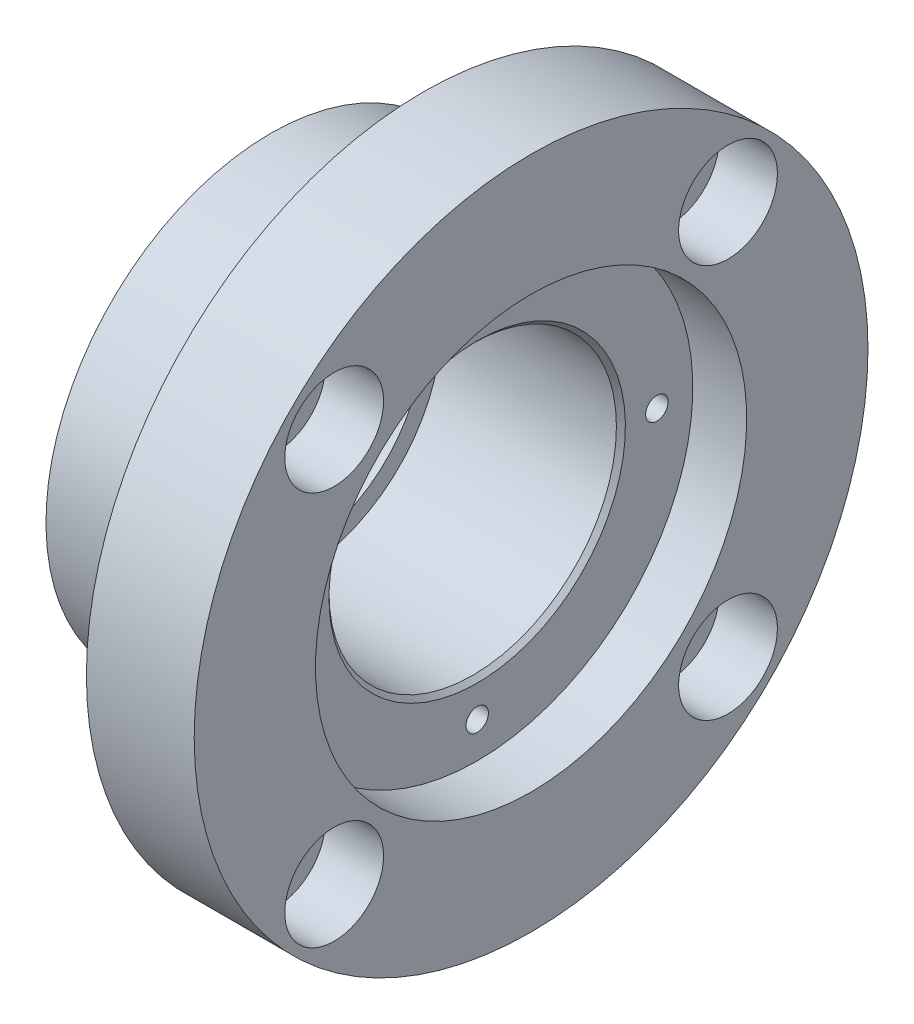
from build123d import *

# Parameters (mm, degrees)
CBORE_SOCKET_HEAD_CAP_SCREW1_D           = 6.6
CBORE_SOCKET_HEAD_CAP_SCREW1_CBORE_D     = 11
CBORE_SOCKET_HEAD_CAP_SCREW1_CBORE_DEPTH = 6.5
TAPPED_HOLE1_D                           = 2.5
TAPPED_HOLE1_DEPTH                       = 8.5
TAPPED_HOLE1_TIP                         = 0.751075774
CHAMFER1_SIZE                            = 0.5


with BuildPart() as part:
    # Sketch1 → Revolve1 (revolve)
    with BuildSketch(Plane.XY):
        Polygon((0, 24), (-6, 24), (-6, 16), (-26, 16), (-26, 14), (-29, 14), (-29, 25), (-12, 25), (-12, 37.5), (0, 37.5), align=None)
    revolve(axis=Axis((0, 0, 0), (-1, 0, 0)))

    # CBORE Socket Head Cap Screw1 (through all)
    with Locations(Plane(origin=(0, 0, 0), x_dir=(0, 0, -1), z_dir=(1, 0, 0))):
        with Locations((-21.920310217, 21.920310217), (21.920310217, 21.920310217), (21.920310217, -21.920310217), (-21.920310217, -21.920310217)):
            CounterBoreHole(CBORE_SOCKET_HEAD_CAP_SCREW1_D / 2, CBORE_SOCKET_HEAD_CAP_SCREW1_CBORE_D / 2, CBORE_SOCKET_HEAD_CAP_SCREW1_CBORE_DEPTH)

    # Tapped Hole1
    with Locations(Plane(origin=(-6, 0, 0), x_dir=(0, 0, -1), z_dir=(1, 0, 0))):
        with Locations((0, 20), (-20, 0), (0, -20), (20, 0)):
            Hole(TAPPED_HOLE1_D / 2, depth=TAPPED_HOLE1_DEPTH)
            with Locations((0, 0, -(TAPPED_HOLE1_DEPTH + TAPPED_HOLE1_TIP / 2))):  # 118° drill point
                Cone(0, TAPPED_HOLE1_D / 2, TAPPED_HOLE1_TIP, mode=Mode.SUBTRACT)

    # Chamfer1
    chamfer1_edges = [part.edges().sort_by_distance(p)[0] for p in [
        (-6, -16, 0),
    ]]
    chamfer(chamfer1_edges, length=CHAMFER1_SIZE)


solid = part.part
